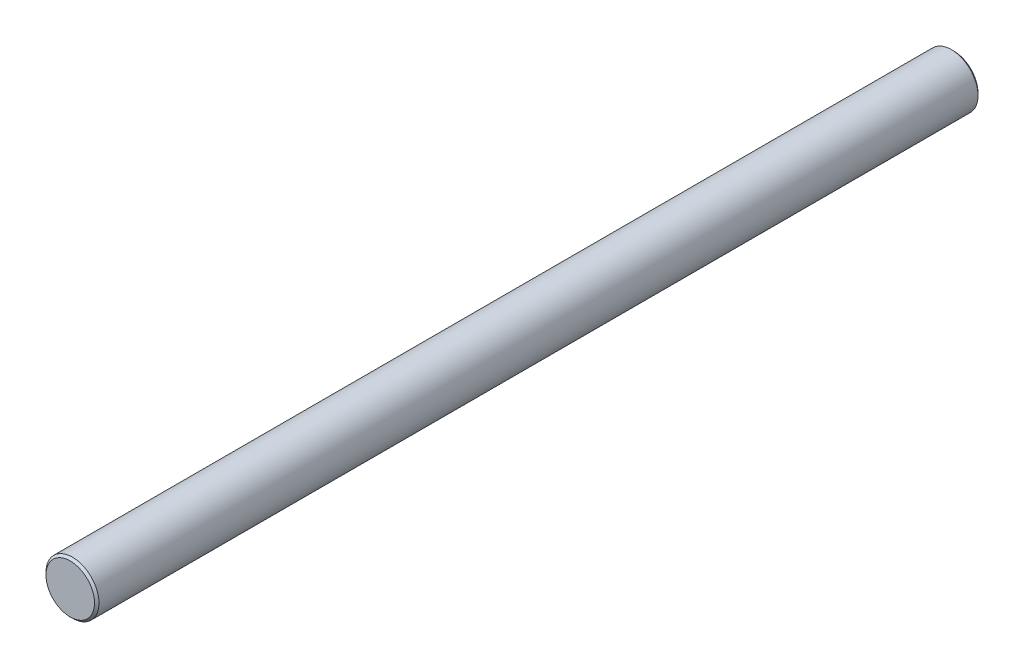
SolidWorks part; units mm, degrees
material "不锈钢 (铁素体)"
ref_plane "前视基准面" through (0, 0, 0) normal (0, 0, 1) x (1, 0, 0)
ref_plane "上视基准面" through (0, 0, 0) normal (0, 1, 0) x (1, 0, 0)
ref_plane "右视基准面" through (0, 0, 0) normal (1, 0, 0) x (0, 0, -1)
sketch "草图1" plane through (0, 0, 0) normal (0, 0, 1) x (1, 0, 0)
  circle A0 centre (0, 0) radius 6
  dimension "D1" = 12
extrude "凸台-拉伸1" add sketch "草图1" along normal mid plane 200
chamfer "倒角1" distance 0.5 angle 45 2 edges at (6, 0, -100) (6, 0, 100)
